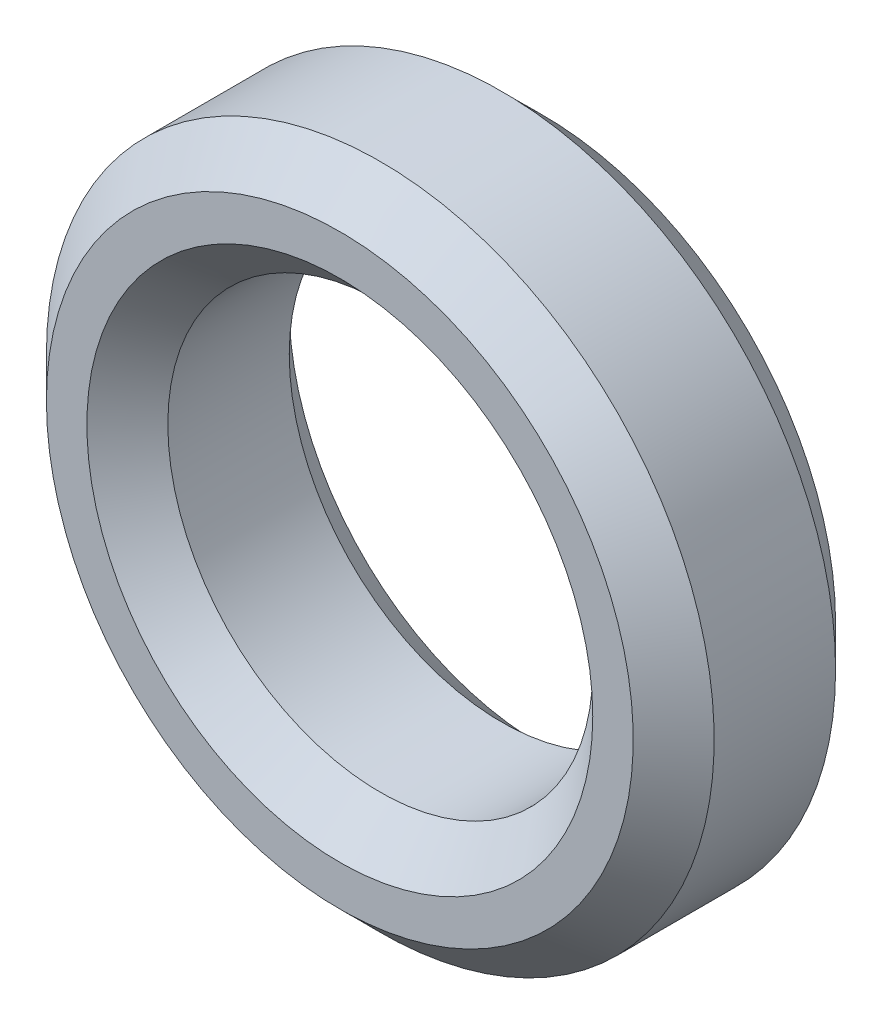
SolidWorks part; units mm, degrees
material "SS41"
ref_plane "Front Plane" through (0, 0, 0) normal (0, 0, 1) x (1, 0, 0)
ref_plane "Top Plane" through (0, 0, 0) normal (0, 1, 0) x (1, 0, 0)
ref_plane "Right Plane" through (0, 0, 0) normal (1, 0, 0) x (0, 0, -1)
sketch "Sketch1" plane through (0, 0, 0) normal (0, 0, 1) x (1, 0, 0)
  circle A0 centre (0, 0) radius 1.65
  circle A1 centre (0, 0) radius 1.05
  dimension "D1" = 2.1
  dimension "D2" = 3.3
extrude "Boss-Extrude1" add sketch "Sketch1" along normal blind 1
chamfer "Chamfer1" distance 0.2 angle 45 4 edges at (1.05, 0, 0) (1.65, 0, 0) (1.05, 0, 1) (1.65, 0, 1)
